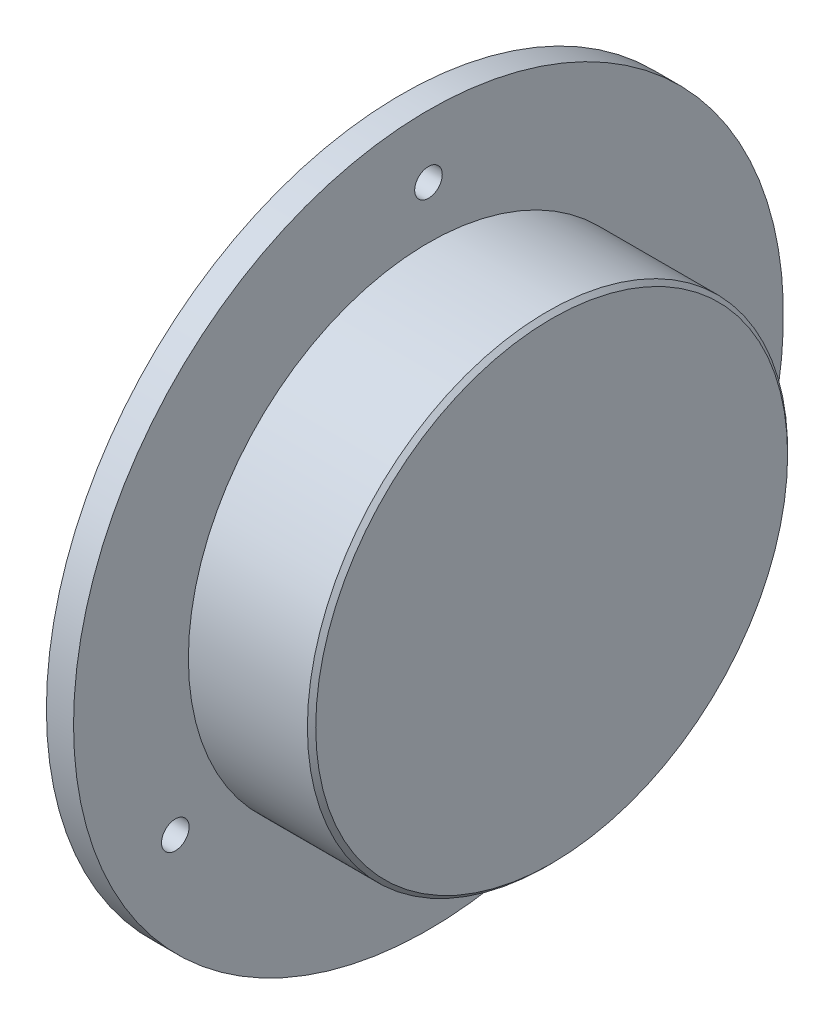
SolidWorks part; units mm, degrees
ref_plane "前视基准面" through (0, 0, 0) normal (0, 0, 1) x (1, 0, 0)
ref_plane "上视基准面" through (0, 0, 0) normal (0, 1, 0) x (1, 0, 0)
ref_plane "右视基准面" through (0, 0, 0) normal (1, 0, 0) x (0, 0, -1)
other "Configuration Table"
sketch "草图2" plane through (0, 0, 0) normal (0, 0, 1) x (1, 0, 0)
  line L0 (0, 0) -> (28.5366, 0) construction
  line L1 (30, 0) -> (30, 50)
  line L2 (30, 50) -> (0, 50)
  line L3 (0, 50) -> (0, 85)
  line L4 (0, 85) -> (6.5, 85)
  line L5 (6.5, 85) -> (6.5, 57.5)
  line L6 (6.5, 57.5) -> (36, 57.5)
  line L7 (36, 57.5) -> (36, 0)
  line L8 (36, 0) -> (30, 0)
  line L9 (30, 0) -> (46.0976, 0) construction
  dimension "D1" = 30
  dimension "D2" = 6.5
  dimension "D3" = 36
  dimension "D4" = 50
  dimension "D5" = 57.5
  dimension "D6" = 85
revolve "旋转1" add sketch "草图2" angle 360 about L0
sketch "草图3" plane through (6.5, 0, 0) normal (1, 0, 0) x (0, 0, -1)
  circle A0 centre (0, 0) radius 70 construction
  point P4 (0, 70)
  point P9 (60.6218, -35)
  point P10 (-60.6218, -35)
  dimension "D1" = 140
  dimension "D3" = 70
  dimension "D4" = 70
  dimension "D2" = 3
hole_wizard "M6 间隙孔1" positions "草图3" profile "草图4" hole size "M6" standard "GB" end condition up to next
sketch "草图4" plane through (6.5, -35, 60.6218) normal (0, 1, 0) x (0, 0, -1)
  line L0 (0, 0) -> (0, 6.5)
  line L1 (0, 6.5) -> (3.3, 6.5)
  line L2 (3.3, 6.5) -> (3.3, 0)
  line L5 (3.3, 0) -> (0, 0)
  line L11 (0, -6.35) -> (0, 107.95) construction
  dimension "通孔孔直径" = 6.6
  dimension "通孔孔深度" = 6.5
chamfer "倒角1" distance 1 angle 45 1 edges at (36, 0, 57.5)
